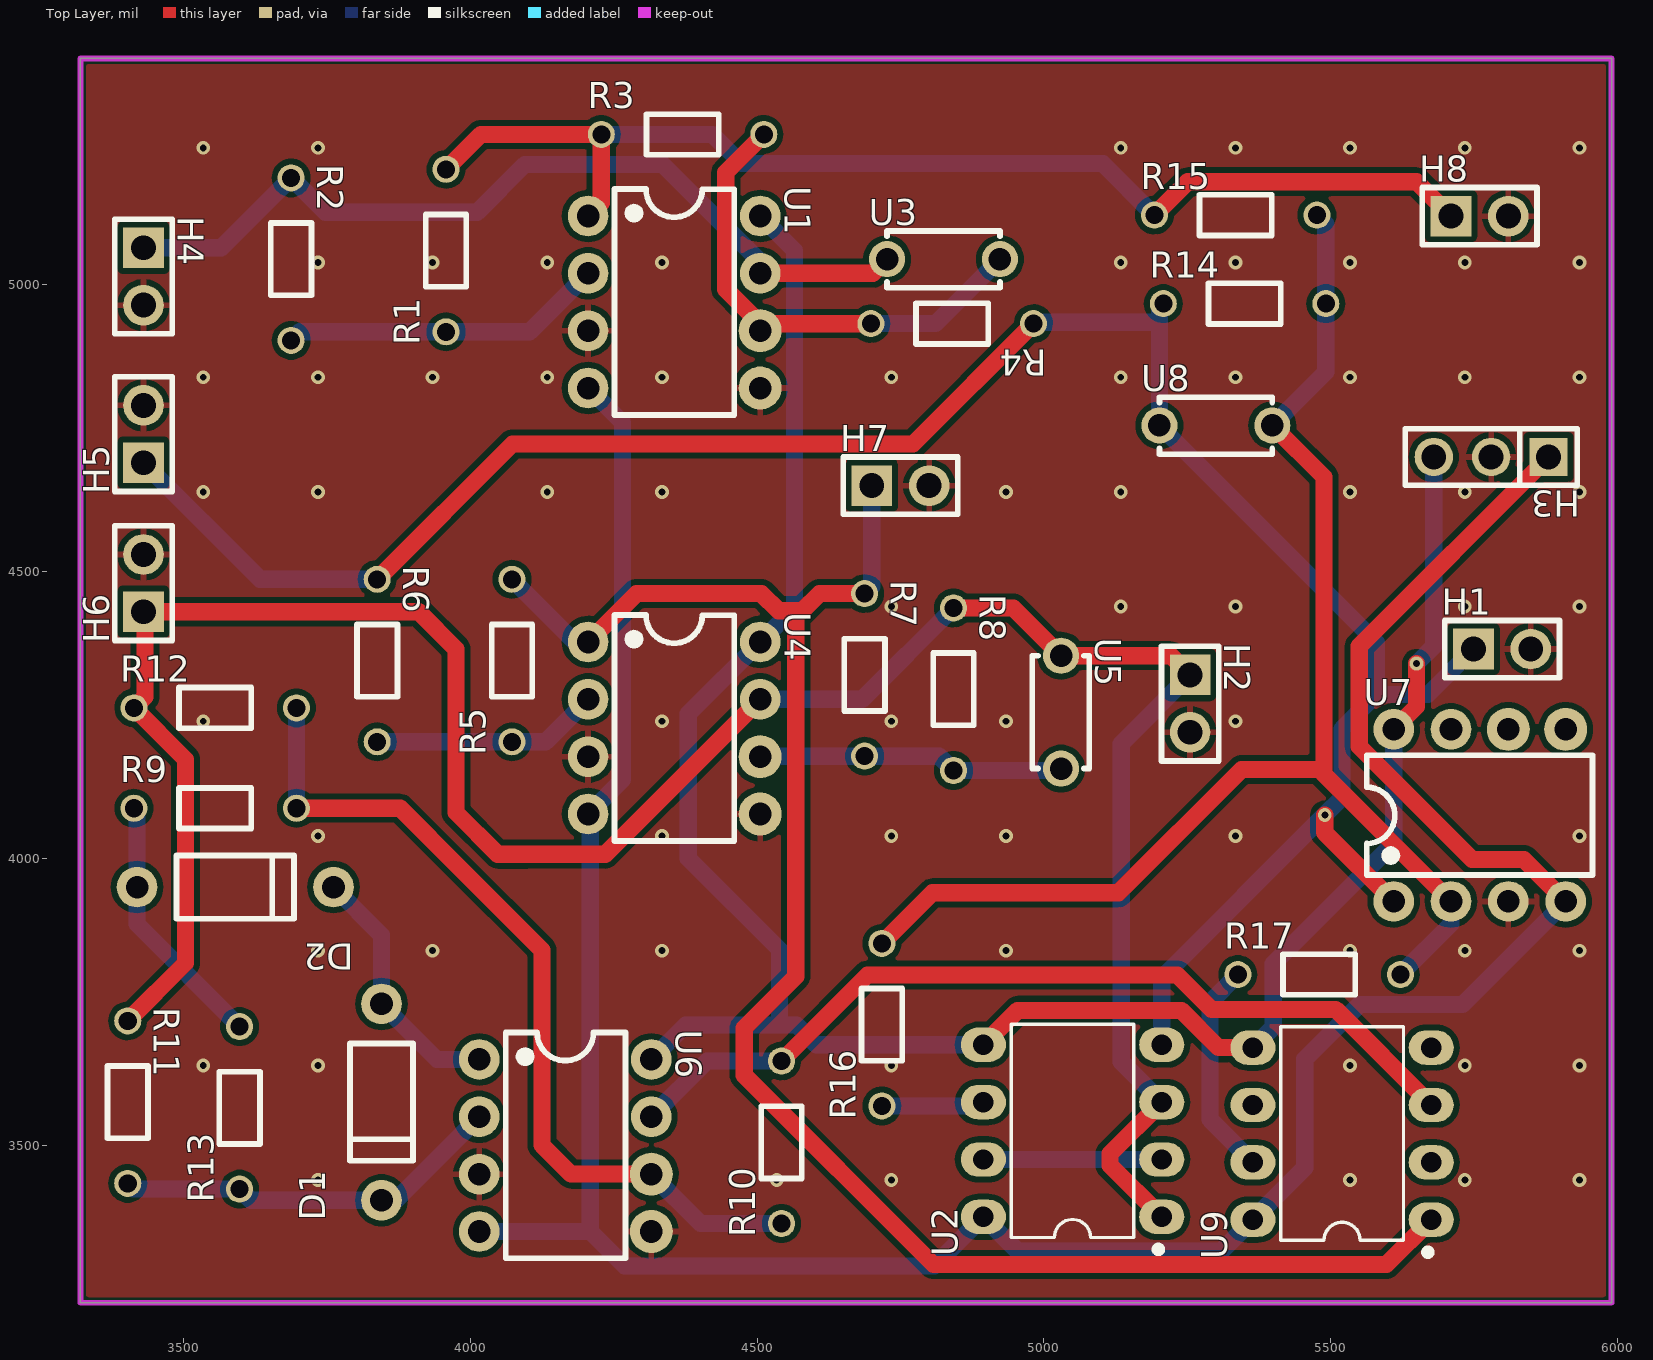
[diagram p0: Top Layer view]
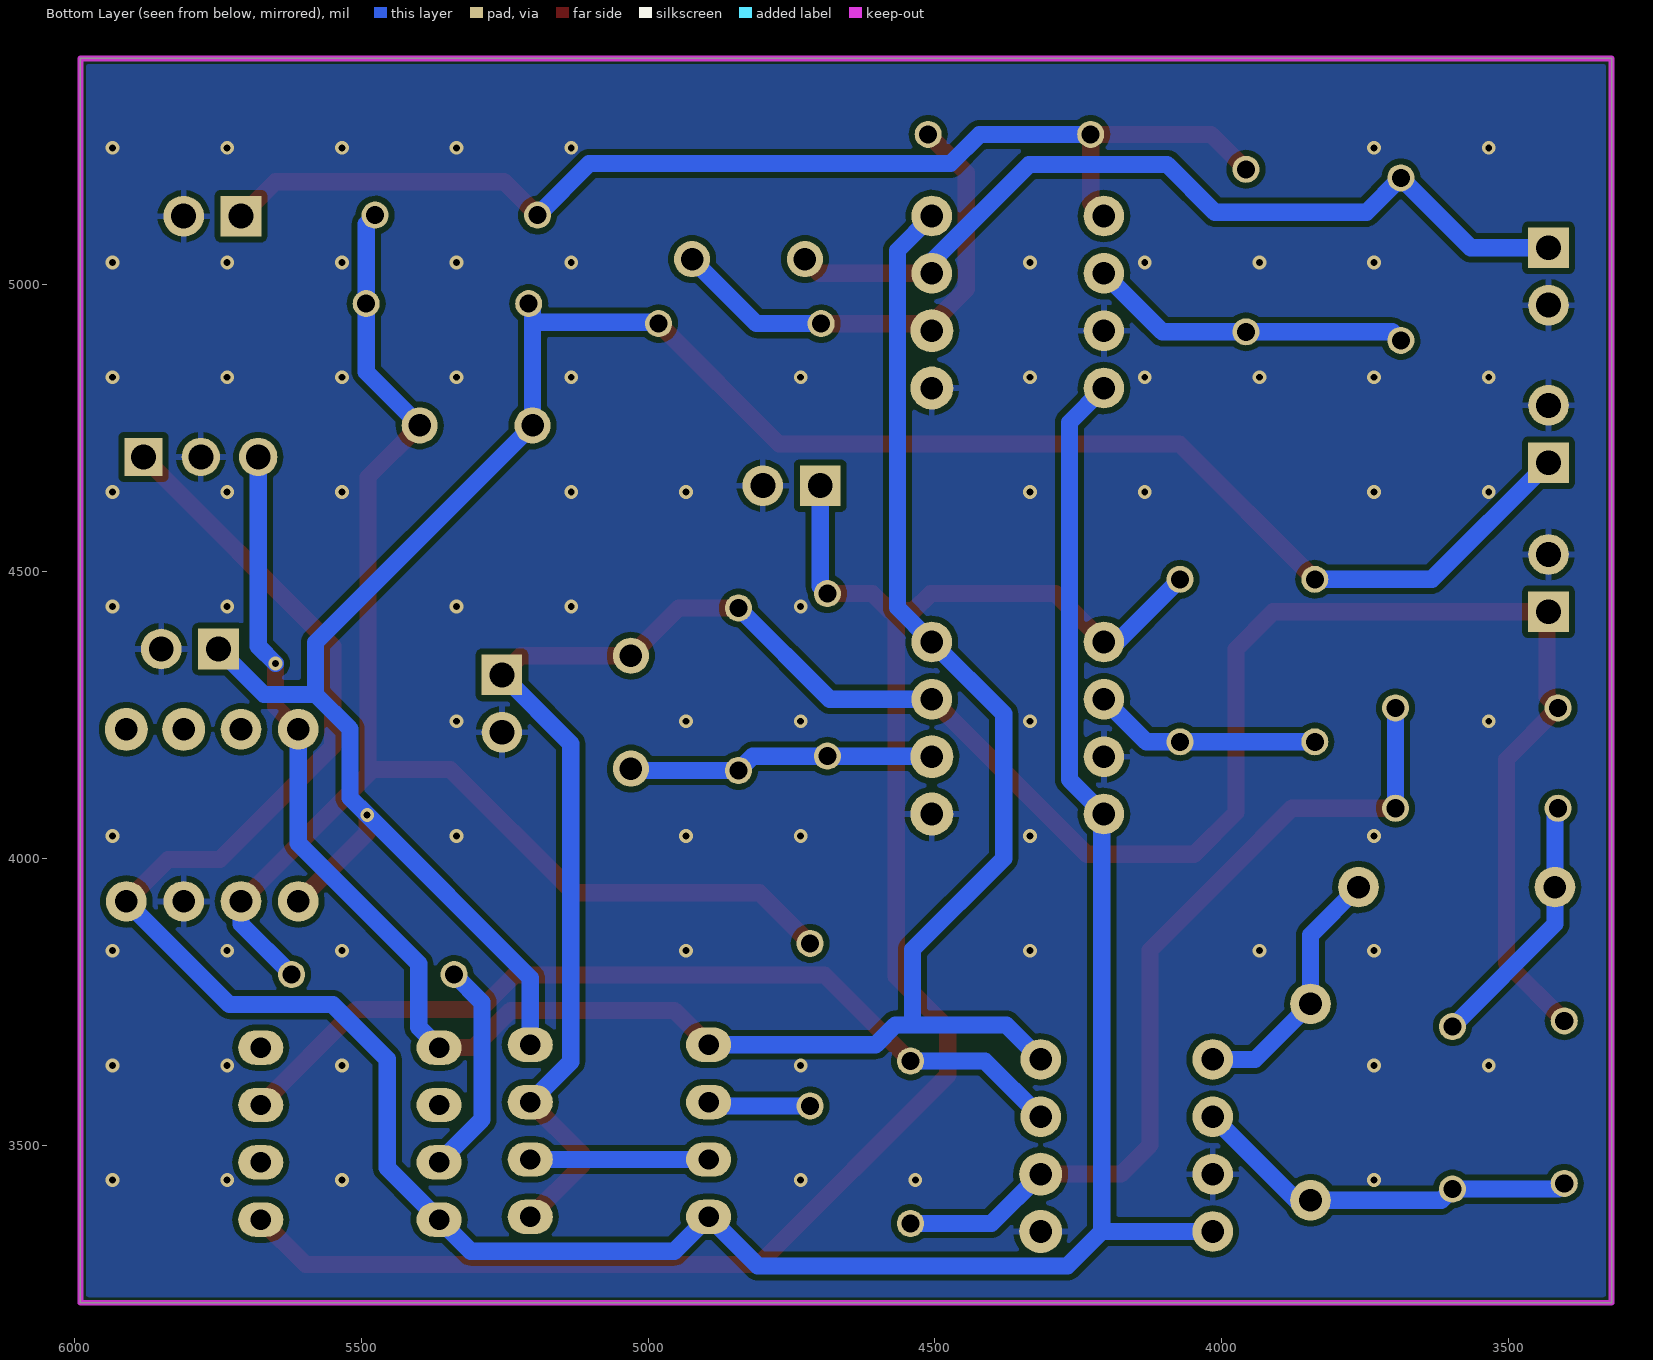
[diagram p1: Bottom Layer view, seen from below]
# Altium PCB MISC51419.pcbdoc
Units mil, origin at the board's own origin, x right, y up, seen from the top; angles counter-clockwise.
Board outline 2670 x 2170 mil, 2 copper layers (Top Layer, Bottom Layer), stack 62.206 mil thick; 36 components, 21 nets, 109 pads, 73 vias.

## Layer stack, top to bottom
Top Solder Mask Layer: solder mask 0.394, Dk 3.3
Top Layer: signal copper 1.379
Dielectric1: surface 59.449, FR4, Dk 4.5
Bottom Layer: signal copper 1.378
Bottom Solder Mask Layer: solder mask 0.394, Dk 3.3

## Board outline
3320,5395 3320,3225 5990,3225 5990,5395

## Design rules (kind name [scope] priority, off if disabled: settings)
BoardOutlineClearance copperThickness2oz_1 [All] p2 off: genericclearance=7.99 ignorepadtopadclearanceinfootprint=FALSE except(0: Arc-SplitContinuation Track-SplitContinuation SMDPad-SplitContinuation THPad-SplitContinuation Via-SplitContinuation Fill-SplitContinuation Region-SplitContinuation Poly-SplitContinuation Text-SplitContinuation Hole-SplitContinuation; 5.98: Arc-CutoutEdge SMDPad-CutoutEdge THPad-CutoutEdge Via-CutoutEdge Fill-CutoutEdge Region-CutoutEdge Text-CutoutEdge; 6.93: Hole-OutlineEdge Hole-CutoutEdge; 10: Poly-OutlineEdge Poly-CutoutEdge; 11.81: Arc-OutlineEdge Track-OutlineEdge SMDPad-OutlineEdge THPad-OutlineEdge Via-OutlineEdge Fill-OutlineEdge Region-OutlineEdge Text-OutlineEdge Track-CutoutEdge)
BoardOutlineClearance copperThickness1oz_1 [All] p4: genericclearance=4.02 ignorepadtopadclearanceinfootprint=FALSE except(0: Arc-SplitContinuation Track-SplitContinuation SMDPad-SplitContinuation THPad-SplitContinuation Via-SplitContinuation Fill-SplitContinuation Region-SplitContinuation Poly-SplitContinuation Text-SplitContinuation Hole-SplitContinuation; 6: SMDPad-CutoutEdge THPad-CutoutEdge Via-CutoutEdge Fill-CutoutEdge Region-CutoutEdge Text-CutoutEdge; 6.93: Hole-OutlineEdge Hole-CutoutEdge; 10: Poly-OutlineEdge Poly-CutoutEdge; 11.8: Arc-OutlineEdge Track-OutlineEdge SMDPad-OutlineEdge THPad-OutlineEdge Via-OutlineEdge Fill-OutlineEdge Region-OutlineEdge Text-OutlineEdge; 11.81: Arc-CutoutEdge Track-CutoutEdge)
Clearance copperThickness2oz [All] p1 off: gap=7.99 ignorepadtopadclearanceinfootprint=FALSE except(5.98: SMDPad-Track SMDPad-SMDPad THPad-Track SMDPad-THPad THPad-THPad Track-Via SMDPad-Via THPad-Via Via-Via Fill-Track Region-Track Fill-SMDPad Region-SMDPad Fill-THPad Region-THPad Fill-Via Region-Via Fill-Fill Fill-Region Region-Region Arc-Track Arc-SMDPad Arc-THPad Arc-Via Fill-Arc Region-Arc Arc-Arc Text-Track SMDPad-Text Text-THPad Text-Via Fill-Text Region-Text Arc-Text Text-Text; 6.93: Hole-Track Hole-SMDPad Hole-THPad Hole-Via Fill-Hole Region-Hole Hole-Arc Hole-Text; 10: Poly-Track Poly-SMDPad Poly-THPad Poly-Via Poly-Fill Poly-Region Poly-Poly Poly-Arc Poly-Text Poly-Hole)
Clearance copperThickness1oz [All] p3: gap=4.02 ignorepadtopadclearanceinfootprint=FALSE except(5.98: SMDPad-Track SMDPad-SMDPad THPad-Track SMDPad-THPad THPad-THPad Track-Via SMDPad-Via THPad-Via Via-Via Fill-Track Region-Track Fill-SMDPad Region-SMDPad Fill-THPad Region-THPad Fill-Via Region-Via Fill-Fill Fill-Region Region-Region; 6: Arc-Track Arc-SMDPad Arc-THPad Arc-Via Fill-Arc Region-Arc Arc-Arc Text-Track SMDPad-Text Text-THPad Text-Via Fill-Text Region-Text Arc-Text Text-Text; 6.93: Hole-Track Hole-SMDPad Hole-THPad Hole-Via Fill-Hole Region-Hole Hole-Arc Hole-Text; 10: Poly-Track Poly-SMDPad Poly-THPad Poly-Via Poly-Fill Poly-Region Poly-Poly Poly-Arc Poly-Text Poly-Hole)
Creepage creepage [All] p1: checkdistance=0 ignoreinternallayers=TRUE applytopolygonpour=TRUE
DiffPairsRouting differentialPair [All] p1: maxlimit=6 minlimit=6 mostfreqgap=6 toplayer_minwidth=5 toplayer_prefwidth=10 toplayer_maxwidth=100 toplayer_mingap=6 toplayer_prefgap=6 toplayer_maxgap=6 bottomlayer_minwidth=5 bottomlayer_prefwidth=10 bottomlayer_maxwidth=100 bottomlayer_mingap=6 bottomlayer_prefgap=6 bottomlayer_maxgap=6 maxuncoupledlength=10
HoleToHoleClearance otherClearance [All] p1: gap=11.81 allowstackedmicrovias=TRUE
Length netLength [All] p1: minlimit=0 maxlimit=0
MatchedLengths netLengthTolerance [All] p1: tolerance=1000
PasteMaskExpansion pasteMaskExpansion [All] p1: expansion=0
PlaneConnect innerPlane [All] p1: planeconnectstyle=Relief reliefexpansion=20 reliefentries=4 reliefconductorwidth=10 reliefairgap=10
PolygonConnect copperRegion [(InNet('GND'))] p1: connectstyle=Relief reliefconductorwidth=10 reliefentries=4 polygonreliefangle="90 Angle" airgapwidth=10 via.connectstyle=Relief via.reliefconductorwidth=10 via.reliefentries=4 via.polygonreliefangle="90 Angle" via.airgapwidth=10
RoutingVias viaSize [All] p1: holewidth=12.01 width=24.02 viastyle="Through Hole" minholewidth=11.81 minwidth=19.68 maxholewidth=248.03 maxwidth=393.7
SolderMaskExpansion solderMaskExpansion [IsVia] p1: expansion=-1000 istentingtop=TRUE
SolderMaskExpansion solderMaskExpansion [All] p2: expansion=2 istentingtop=FALSE
Width copperThickness2oz_2 [All] p1 off: maxlimit=100 minlimit=8 preferedwidth=10
Width copperThickness1oz_2 [All] p2: maxlimit=10 minlimit=10 preferedwidth=10 toplayer_minwidth=30 toplayer_maxwidth=100 toplayer_prefwidth=30 bottomlayer_minwidth=30 bottomlayer_maxwidth=100 bottomlayer_prefwidth=30

## Components (designator, comment, footprint, x,y, rotation, side; value= is the part's Value field where it differs from the comment)
D1 "" DO_1N4007 3845,3575 r90 top
D2 "" DO_1N4007 3590,3950 r180 top
H1 "" HDR-TH_2P-P2.54-V-M-1 5799.17,4365.06 r0 top
H2 "" HDR-TH_2P-P2.54-V-M-1 5255,4270 r270 top
H3 "" HDR-TH_3P-P2.54-V-M 5780,4700 r180 top
H4 "" HDR-TH_2P-P2.54-V-M-1 3430,5014.75 r270 top
H5 "" HDR-TH_2P-P2.54-V-M-1 3430,4740 r90 top
H6 "" HDR-TH_2P-P2.54-V-M-1 3430,4480 r90 top
H7 "" HDR-TH_2P-P2.54-V-M-1 4750,4650 r0 top
H8 "" HDR-TH_2P-P2.54-V-M-1 5760,5120 r0 top
R1 "10kΩ" Res_1/8W 3960,5060 r90 top
R2 "10kΩ" Res_1/8W 3685,5045 r270 top
R3 "50kΩ" Res_1/8W 4370,5260 r0 top
R4 "18.1kΩ" Res_1/8W 4840,4935 r180 top
R5 "10kΩ" Res_1/8W 4075,4345 r90 top
R6 "10kΩ" Res_1/8W 3835,4345 r270 top
R7 "10kΩ" Res_1/8W 4685,4320 r270 top
R8 "40kΩ" Res_1/8W 4840,4295 r270 top
R9 "5kΩ" Res_1/8W 3555,4085 r0 top
R10 "10kΩ" Res_1/8W 4545,3505 r90 top
R11 "10kΩ" Res_1/8W 3400,3575 r270 top
R12 "10kΩ" Res_1/8W 3555,4260 r0 top
R13 "10kΩ" Res_1/8W 3600,3565 r90 top
R14 "71.68kΩ" Res_1/8W 5350,4965 r0 top
R15 "40kΩ" Res_1/8W 5334.49,5119.24 r0 top
R16 "567Ω" Res_1/8W 4720,3710 r90 top
R17 "2.67KΩ" Res_1/8W 5480,3795 r0 top
U1 "TL082CN(LX)" PDIP-8_L9.6-W6.4-P2.54-LS7.6-BL 4355.27,4970.23 r270 top
U2 "AD633ANZ" PDIP-8_L9.3-W6.4-P2.54-LS7.9-BL-1 5050,3525 r90 top
U3 "10nF" CAP-TH_L5.0-W2.5-P5.00-D1.0 4825,5045 r0 top
U4 "TL082CN(LX)" PDIP-8_L9.6-W6.4-P2.54-LS7.6-BL 4355.27,4227.39 r270 top
U5 "10nF" CAP-TH_L5.0-W2.5-P5.00-D1.0 5030,4255 r270 top
U6 "TL082CN(LX)" PDIP-8_L9.6-W6.4-P2.54-LS7.6-BL 4165.54,3499.41 r270 top
U7 "TL082CN(LX)" PDIP-8_L9.6-W6.4-P2.54-LS7.6-BL 5760,4075 r0 top
U8 "10nF" CAP-TH_L5.0-W2.5-P5.00-D1.0 5300,4755 r0 top
U9 "AD633ANZ" PDIP-8_L9.3-W6.4-P2.54-LS7.9-BL-1 5520,3520 r90 top

## Footprints (in the part's own frame and the unit in brackets; to place one, negate y for a bottom-side part, rotate by r counter-clockwise, add the part's x,y. Pads: shape width x height; smd on the part's side, far side on the other; paste and mask are expansions set on the pad)
CAP-TH_L5.0-W2.5-P5.00-D1.0 [mm]
  round 1.6 hole 1: 1(-2.5,0) 2(2.5,0)
  silkscreen extent -2.5,-1.27 2.5,1.25
DO_1N4007 [mm]
  round 1.8 hole 1 paste+0 mask+0.051: 1(-4.35,0) 2(4.35,0)
  silkscreen extent -2.6,-1.4 2.6,1.4
HDR-TH_2P-P2.54-V-M-1 [mm]
  rect 1.8x1.8 hole 1.1: 1(-1.27,0)
  round 1.8 hole 1.1: 2(1.27,0)
  silkscreen extent -2.54,-1.27 2.54,1.27
HDR-TH_3P-P2.54-V-M [mm]
  rect 1.7x1.7 hole 1.1: 1(-2.54,0)
  round 1.7 hole 1.1: 2(0,0) 3(2.54,0)
  silkscreen extent -3.81,-1.25 3.81,1.25
PDIP-8_L9.3-W6.4-P2.54-LS7.9-BL-1 [mm]
  oval 1.524x2 hole 0.9: 1(-3.81,-3.95) 2(-1.27,-3.95) 3(1.27,-3.95) 4(3.81,-3.95) 5(3.81,3.95) 6(1.27,3.95) 7(-1.27,3.95) 8(-3.81,3.95)
  silkscreen extent -5.4,-3.95 4.73,2.72
PDIP-8_L9.6-W6.4-P2.54-LS7.6-BL [mm]
  round 1.8 hole 1: 1(-3.81,-3.81) 2(-1.27,-3.81) 3(1.27,-3.81) 4(3.81,-3.81) 7(-1.27,3.81) 8(-3.81,3.81)
  round 1.905 hole 1: 5(3.81,3.81) 6(1.27,3.81)
  silkscreen extent -5,-2.64 5,2.67
Res_1/8W [mil]
  round 47.2 hole 31.5 paste+0 mask+2: 1(-141.7,2.48) 2(141.7,2.48)
  silkscreen extent -63,-33 63,38

## Via types
v1: diameter 24.02, hole 12, Top Layer to Bottom Layer, 73 vias

## Nets (pads, with @x,y where several pads share a name; then routed paths per layer and width w, separated by ;. In a path a pad name is that pad's centre, name@x,y a point inside that pad or via, vN(x,y) a via of type N, cw(c..) or ccw(c..) an arc to the next point about the centre after c; other vN are vias at no path point)
$1N4: R1.1 R2.2 U1.2 | length 566.2
  Bottom Layer w30: R2.2 3702.47,4918.3 R1.1 4103.34,4918.3 U1.2
$1N8: R3.2 R4.2 U1.6 U3.2 | length 859.3
  Top Layer w30: U1.6 U1.6@4505.27,4932.48 ; R3.2 4445.27,5196.04 4445.27,4992.48 U1.6@4505.27,4932.48 ; R4.2 U1.6@4505.27,4932.48
  Bottom Layer w30: R4.2 4810.95,4932.53 U3.2
$1N15: R7.2 R8.2 U4.6 U5.2 | length 536.8
  Bottom Layer w30: U4.6 4506.17,4178.3 R7.2 4817.48,4178.3 R8.2 5026.72,4153.3 U5.2
$1N19: R5.1 R6.2 U4.2 | length 398.5
  Bottom Layer w30: R6.2 R5.1 4131.17,4203.3 U4.2
$1N26: D1.1 R11.2 R13.1 U6.2 | length 685.6
  Bottom Layer w30: R11.2 3412.48,3423.3 R13.1 3617.08,3403.74 D1.1 3869.86,3403.74 U6.2
$1N31: R9.2 R10.1 R12.2 U6.6 | length 1520
  Top Layer w30: R9.2 3877.52,4087.48 3982.48,3982.52 4125,3840 4125,3500 4175.59,3449.41 U6.6
  Bottom Layer w30: R9.2 R12.2 ; U6.6 4401.65,3363.3 R10.1
$1N32: D1.2 D2.1 U6.1 | length 449.1
  Bottom Layer w30: D2.1 3845,3866.26 D1.2 3941.84,3649.41 U6.1
$1N33: D2.2 R9.1 R13.2 | length 457.1
  Bottom Layer w30: R9.1 3418.74,4082.03 D2.2 3418.74,3885.48 R13.2
$1N34: R10.2 U6.7 U9.3 | length 1556.3
  Top Layer w30: R10.2 4692.52,3796.7 5232.52,3796.7 5292.52,3736.7 5508.81,3736.7 U9.3
  Bottom Layer w30: U6.7 4412.82,3646.7 R10.2
$1N38: R14.2 R15.2 R16.2 R17.2 U7.2 U8.2 | length 2431.5
  Top Layer w30: R16.2 4805.82,3940 5130,3940 5345,4155 5488.42,4155 ; U8.2 5488.42,4665 5488.42,4155 ; U7.2 5488.42,4146.57 5488.42,4155
  Bottom Layer w30: U8.2 5491.7,4848.28 R14.2 5491.7,5106.2 R15.2 ; R17.2 5710,3885.78 U7.2
$1N49: U2.2 U2.7 | length 311
  Bottom Layer w30: U2.7 U2.2
$1N51: R16.1 U2.6 | length 179.7
  Bottom Layer w30: R16.1 4887.79,3568.3 U2.6
$1N58: R17.1 U9.7 | length 378.3
  Bottom Layer w30: R17.1 5290,3749.18 5290,3544.49 U9.7
-X: H7.1 R5.2 R7.1 U4.1 U9.1 | length 3127.9
  Top Layer w30: U4.1 4289.58,4461.7 4507.48,4461.7 4537.48,4431.7 4567.48,4431.7 ; R7.1 4608.74,4461.7 4578.74,4431.7 4567.48,4431.7 ; U9.1 5597.21,3291.7 4807.48,3291.7 4477.48,3621.7 4477.48,3704.22 4567.48,3794.22 4567.48,4431.7
  Bottom Layer w30: R5.2 4181.83,4377.39 U4.1 ; R7.1 4700,4474.22 H7.1
-Y: H8.1 R1.2 R3.1 R15.1 U1.1 | length 2036.7
  Top Layer w30: R1.2 4018.3,5262.48 R3.1 4228.3,5143.26 U1.1 ; R15.1 5251.07,5180 5650,5180 H8.1
  Bottom Layer w30: R3.1 4422.02,5262.48 4472.79,5211.71 5102.79,5211.71 R15.1
GND: H1.2 H2.2 H3.2 H4.2 H5.2 H6.2 H7.2 H8.2 U1.3 U1.5 U4.3 U4.5 U6.3 U6.5 U7.3
  other v1: 3734.1,3439.1 4534.1,3439.1 4734.1,3439.1 5534.1,3439.1 5734.1,3439.1 5934.1,3439.1 3534.1,3639.1 3734.1,3639.1 4734.1,3639.1 5534.1,3639.1 5734.1,3639.1 5934.1,3639.1 3734.1,3839.1 3934.1,3839.1 4334.1,3839.1 4934.1,3839.1 5534.1,3839.1 5734.1,3839.1 5934.1,3839.1 3734.1,4039.1 4334.1,4039.1 4734.1,4039.1 4934.1,4039.1 5334.1,4039.1 5934.1,4039.1 3534.1,4239.1 4334.1,4239.1 4734.1,4239.1 4934.1,4239.1 5334.1,4239.1 4734.1,4439.1 5134.1,4439.1 5334.1,4439.1 5734.1,4439.1 5934.1,4439.1 3534.1,4639.1 3734.1,4639.1 4134.1,4639.1 4334.1,4639.1 4934.1,4639.1 5134.1,4639.1 5534.1,4639.1 5734.1,4639.1 5934.1,4639.1 3534.1,4839.1 3734.1,4839.1 3934.1,4839.1 4134.1,4839.1 4334.1,4839.1 4734.1,4839.1 5134.1,4839.1 5334.1,4839.1 5534.1,4839.1 5734.1,4839.1 5934.1,4839.1 3734.1,5039.1 3934.1,5039.1 4134.1,5039.1 4334.1,5039.1 5134.1,5039.1 5334.1,5039.1 5534.1,5039.1 5734.1,5039.1 5934.1,5039.1 3534.1,5239.1 3734.1,5239.1 5134.1,5239.1 5334.1,5239.1 5534.1,5239.1 5734.1,5239.1 5934.1,5239.1
VCC: H3.1 U1.4 U2.8 U4.4 U6.4 U7.4 U9.8 | length 4978.8
  Top Layer w30: H3.1 5550,4370 5550,4195 5747.03,3997.97 5837.03,3997.97 U7.4
  Bottom Layer w30: U6.4 4208.9,3349.41 ; U1.4 4265.27,4760.23 4265.27,4137.39 U4.4 4208.9,4073.76 4208.9,3349.41 ; U7.4 5730,3745 5550,3745 5455,3650 5455,3460.51 U9.8 5309.49,3315 4954.49,3315 U2.8 4808.9,3289.41 4268.9,3289.41 4208.9,3349.41
VEE: H3.3 U1.8 U2.5 U4.8 U6.8 U7.8 U9.5 | length 3878.8
  Top Layer w30: U2.5 4954.49,3735 5239.49,3735 5304.49,3670 U9.5 ; U7.8 5650,4265 v1(5650,4340)
  Bottom Layer w30: U6.8 4375.54,3709.41 4538.9,3709.41 ; U1.8 4565.27,5060.23 4565.27,4437.39 U4.8 4380,4252.12 4380,4183.96 4380,4000 4538.9,3841.1 4538.9,3709.41 ; U2.5 4603.32,3675 4568.9,3709.41 4538.9,3709.41 ; U9.5 5400,3705.51 5400,3816.26 5610,4026.26 U7.8 ; v1(5650,4340) 5680,4370 H3.3
X: H1.1 H5.1 R4.1 R6.1 R14.1 U2.4 U7.1 U8.1 | length 4051.2
  Top Layer w30: R6.1 4073.3,4722.53 4771.7,4722.53 R4.1 ; v1(5490,4075.89) 5490,4045 U7.1
  Bottom Layer w30: H5.1 3633.3,4486.7 R6.1 ; R4.1 4984.18,4935 5201.57,4935 ; U2.4 5205.51,3791.4 v1(5490,4075.89) 5520,4105.89 5520,4225.89 5580,4285.89 ; R14.1 5201.57,4960.75 5201.57,4935 ; H1.1 5670,4285.89 5580,4285.89 ; 5201.57,4935 U8.1 5580,4376.58 5580,4285.89
Y: H4.1 R2.1 U1.7 U3.1 | length 1507.2
  Top Layer w30: U1.7 4701.81,5020.23 U3.1
  Bottom Layer w30: H4.1 3565.52,5064.75 R2.1 3747.47,5126.7 4011.7,5126.7 4095,5210 4335.72,5210 4505.27,5040.45 U1.7
Z: H2.1 H6.1 R8.1 R11.1 R12.1 U2.1 U2.3 U4.7 U5.1 | length 4297.5
  Top Layer w30: R11.1 3503.3,3817.52 3503.3,4172.48 R12.1 3432.61,4281.78 3432.61,4427.39 H6.1@3440.31,4430 ; H6.1 H6.1@3440.31,4430 ; U4.7 4235.27,4007.39 4099.81,4007.39 4047.61,4007.39 3975,4080 3975,4365 3910,4430 H6.1@3440.31,4430 ; R8.1 4946.73,4436.7 U5.1 5221.57,4353.43 H2.1 ; U2.1 5115.51,3465 5115.51,3485 U2.3
  Bottom Layer w30: U4.7 4683.17,4277.39 R8.1 ; U2.3 5135,3645.51 5135,4200 H2.1
pads on no net: U7.5 U7.6 U7.7 U9.2 U9.4 U9.6

## Polygon pours and split planes (outlines as drawn)
GND on Bottom Layer (solid, remove dead copper, pour order 2): 3000,5605 3000,3085 6365,3085 6365,5605
GND on Top Layer (solid, remove dead copper, pour order 0): 3130,5490 3130,3000 6320,3000 6320,5490

## Keep-outs
Board Outline Layer:
  the board outline again, w10